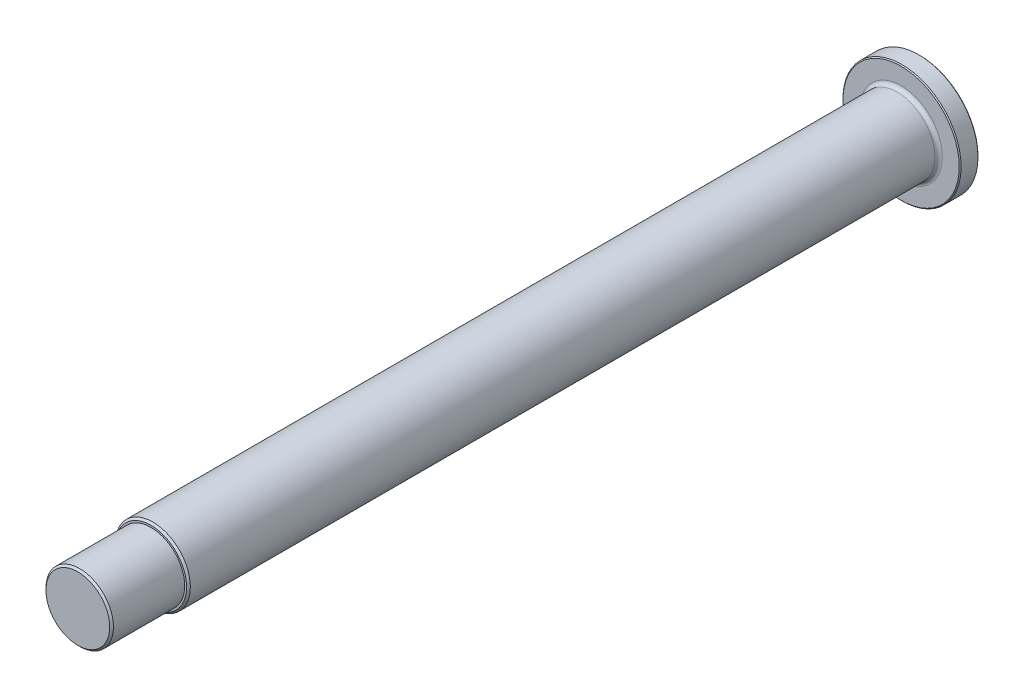
SolidWorks part; units mm, degrees
material "普通碳钢"
ref_plane "前视" through (0, 0, 0) normal (0, 0, 1) x (1, 0, 0)
ref_plane "上视" through (0, 0, 0) normal (0, 1, 0) x (1, 0, 0)
ref_plane "右视" through (0, 0, 0) normal (1, 0, 0) x (0, 0, -1)
sketch "草图1" plane through (0, 0, 0) normal (0, 0, 1) x (1, 0, 0)
  line L0 (-79.9655, 0) -> (85.3903, 0) construction
  line L1 (0, 50.8323) -> (0, -54.6498) construction
  circle A0 centre (0, 0) radius 31.5
  dimension "D1" = 63
extrude "凸台-拉伸1" add sketch "草图1" along normal blind 10
sketch "草图2" plane through (0, 0, 10) normal (0, 0, 1) x (1, 0, 0)
  circle A0 centre (0, 0) radius 20
  dimension "D1" = 40
extrude "凸台-拉伸2" add sketch "草图2" along normal blind 400
sketch "草图3" plane through (0, 0, 410) normal (0, 0, 1) x (1, 0, 0)
  circle A0 centre (0, 0) radius 18
  dimension "D1" = 36
extrude "凸台-拉伸3" add sketch "草图3" along normal blind 39
fillet "圆角1" radius 2 1 edges at (20, 0, 10)
chamfer "倒角2" distance 1 angle 45 2 edges at (18, 0, 449) (20, 0, 410)
chamfer "倒角3" distance 0.5 angle 45 2 edges at (31.5, 0, 10) (31.5, 0, 0)
